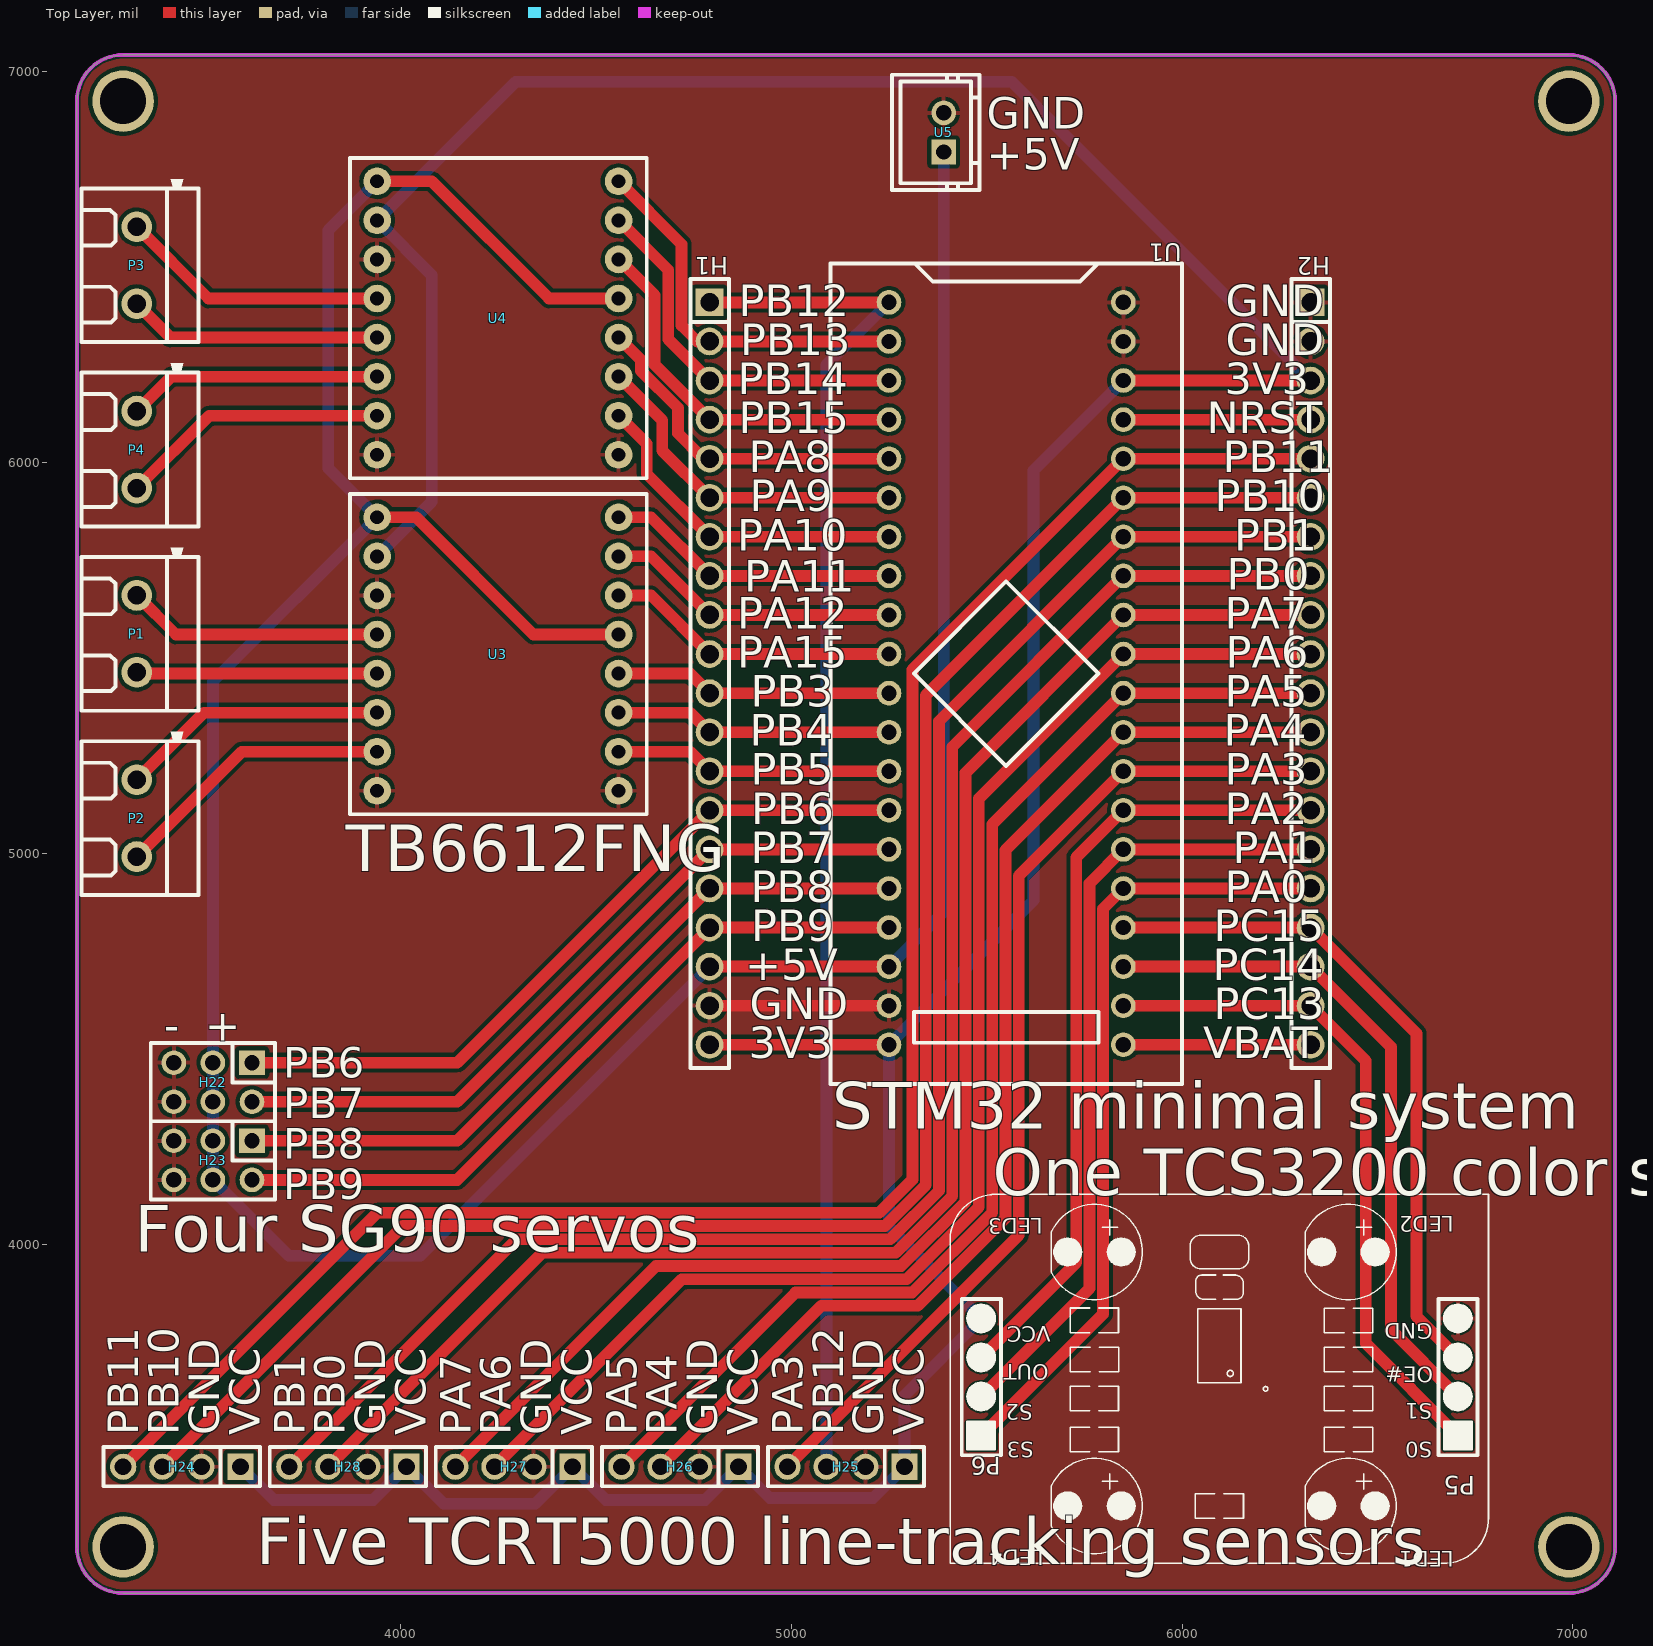
[diagram p0: Top Layer view]
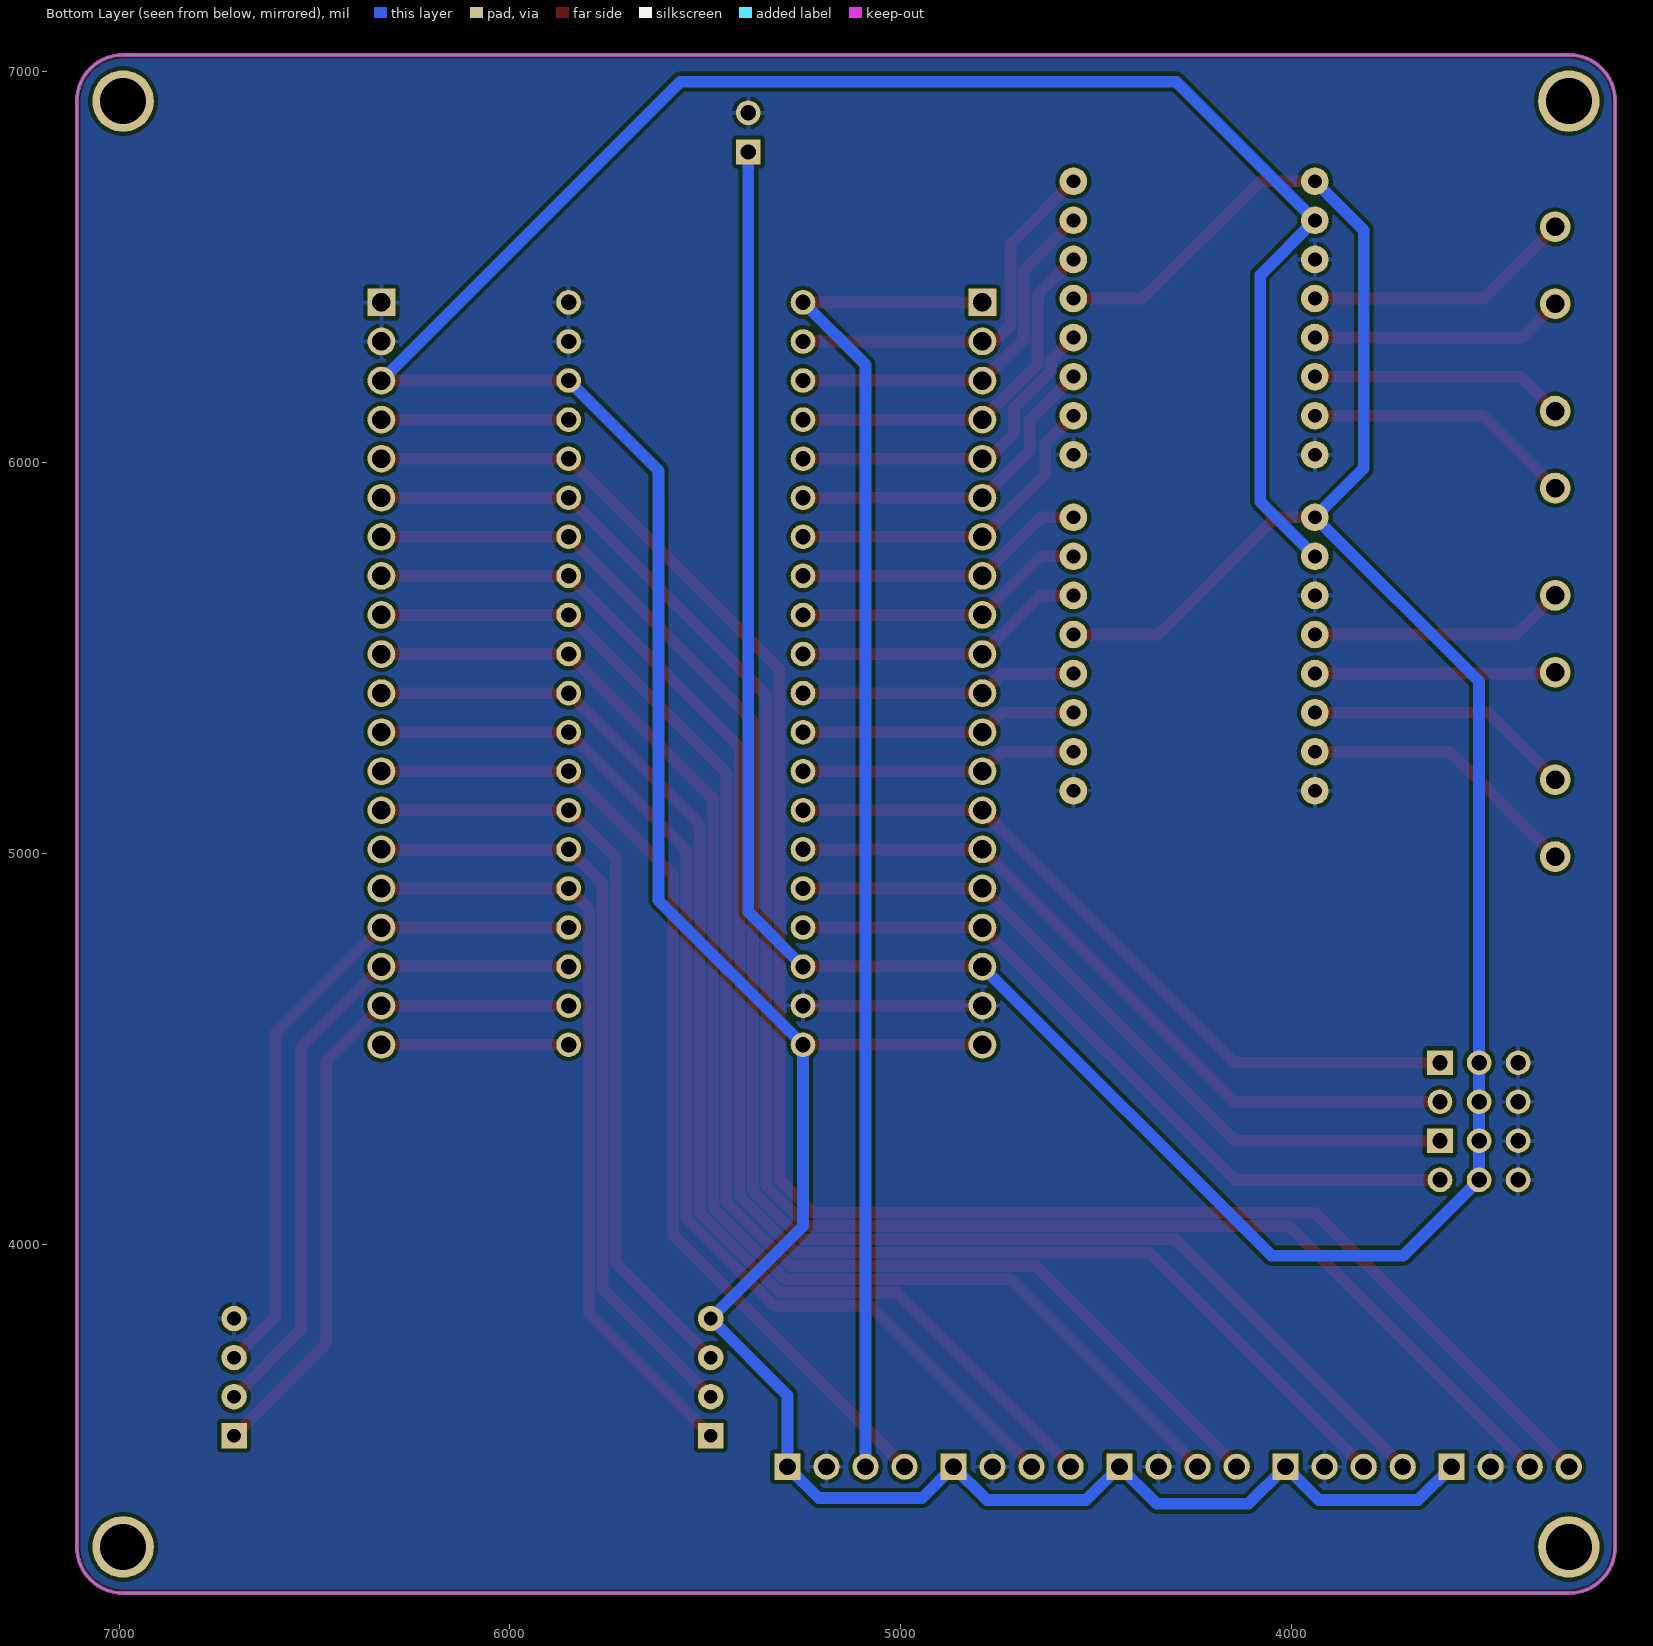
[diagram p1: Bottom Layer view, seen from below]
# Altium PCB MISC88999.pcbdoc
Units mil, origin at the board's own origin, x right, y up, seen from the top; angles counter-clockwise.
Board outline 3937.01 x 3937.01 mil, 2 copper layers (Top Layer, Bottom Layer), stack 62.206 mil thick; 19 components, 45 nets, 166 pads, 0 vias.

## Layer stack, top to bottom
Top Solder Mask Layer: solder mask 0.394, Dk 3.3
Top Layer: signal copper 1.379
Dielectric1: surface 59.449, FR4, Dk 4.5
Bottom Layer: signal copper 1.378
Bottom Solder Mask Layer: solder mask 0.394, Dk 3.3

## Board outline
6990.39,3106.5 ccw(c6990.39,3224.61) 7108.5,3224.61 7108.5,6925.39 ccw(c6990.39,6925.39) 6990.39,7043.5 3289.61,7043.5 ccw(c3289.61,6925.39) 3171.5,6925.39 3171.5,3224.61 ccw(c3289.61,3224.61) 3289.61,3106.5

## Design rules (kind name [scope] priority, off if disabled: settings)
BoardOutlineClearance copperThickness2oz_1 [All] p2 off: genericclearance=7.99 ignorepadtopadclearanceinfootprint=FALSE except(0: Arc-SplitContinuation Track-SplitContinuation SMDPad-SplitContinuation THPad-SplitContinuation Via-SplitContinuation Fill-SplitContinuation Region-SplitContinuation Poly-SplitContinuation Text-SplitContinuation Hole-SplitContinuation; 5.98: Arc-CutoutEdge Track-CutoutEdge SMDPad-CutoutEdge THPad-CutoutEdge Via-CutoutEdge Text-CutoutEdge; 6.9: Hole-OutlineEdge Hole-CutoutEdge; 10: Poly-OutlineEdge Poly-CutoutEdge; 11.81: Arc-OutlineEdge Track-OutlineEdge SMDPad-OutlineEdge THPad-OutlineEdge Via-OutlineEdge Fill-OutlineEdge Region-OutlineEdge Text-OutlineEdge Fill-CutoutEdge Region-CutoutEdge)
BoardOutlineClearance Plane_innerPlane_1 [All] p4 off: genericclearance=4.02 ignorepadtopadclearanceinfootprint=FALSE except(0: Arc-SplitContinuation Track-SplitContinuation SMDPad-SplitContinuation THPad-SplitContinuation Via-SplitContinuation Fill-SplitContinuation Region-SplitContinuation Poly-SplitContinuation Text-SplitContinuation Hole-SplitContinuation; 5.98: Arc-CutoutEdge Track-CutoutEdge SMDPad-CutoutEdge THPad-CutoutEdge Via-CutoutEdge Text-CutoutEdge; 6.9: Hole-OutlineEdge Hole-CutoutEdge; 10: Poly-OutlineEdge Poly-CutoutEdge; 11.81: Arc-OutlineEdge Track-OutlineEdge SMDPad-OutlineEdge THPad-OutlineEdge Via-OutlineEdge Fill-OutlineEdge Region-OutlineEdge Text-OutlineEdge Fill-CutoutEdge Region-CutoutEdge)
BoardOutlineClearance Copper_copperRegion_1 [All] p6 off: genericclearance=4.02 ignorepadtopadclearanceinfootprint=FALSE except(0: Arc-SplitContinuation Track-SplitContinuation SMDPad-SplitContinuation THPad-SplitContinuation Via-SplitContinuation Fill-SplitContinuation Region-SplitContinuation Poly-SplitContinuation Text-SplitContinuation Hole-SplitContinuation; 5.98: Arc-CutoutEdge Track-CutoutEdge SMDPad-CutoutEdge THPad-CutoutEdge Via-CutoutEdge Text-CutoutEdge; 6.9: Hole-OutlineEdge Hole-CutoutEdge; 10: Poly-OutlineEdge Poly-CutoutEdge; 11.81: Arc-OutlineEdge Track-OutlineEdge SMDPad-OutlineEdge THPad-OutlineEdge Via-OutlineEdge Fill-OutlineEdge Region-OutlineEdge Text-OutlineEdge Fill-CutoutEdge Region-CutoutEdge)
BoardOutlineClearance copperThickness1oz_1 [All] p8: genericclearance=4.02 ignorepadtopadclearanceinfootprint=FALSE except(0: Arc-SplitContinuation Track-SplitContinuation SMDPad-SplitContinuation THPad-SplitContinuation Via-SplitContinuation Fill-SplitContinuation Region-SplitContinuation Poly-SplitContinuation Text-SplitContinuation Hole-SplitContinuation; 5.98: Arc-CutoutEdge Track-CutoutEdge SMDPad-CutoutEdge THPad-CutoutEdge Via-CutoutEdge Text-CutoutEdge; 6.9: Hole-OutlineEdge Hole-CutoutEdge; 10: Poly-OutlineEdge Poly-CutoutEdge; 11.81: Arc-OutlineEdge Track-OutlineEdge SMDPad-OutlineEdge THPad-OutlineEdge Via-OutlineEdge Fill-OutlineEdge Region-OutlineEdge Text-OutlineEdge Fill-CutoutEdge Region-CutoutEdge)
Clearance copperThickness2oz [All] p1 off: gap=7.99 ignorepadtopadclearanceinfootprint=FALSE except(5.98: SMDPad-Track SMDPad-SMDPad THPad-Track SMDPad-THPad THPad-THPad Track-Via SMDPad-Via THPad-Via Via-Via Fill-SMDPad Region-SMDPad Fill-THPad Region-THPad Fill-Via Region-Via Fill-Fill Fill-Region Region-Region Arc-Track Arc-SMDPad Arc-THPad Arc-Via Fill-Arc Region-Arc Arc-Arc Text-Track SMDPad-Text Text-THPad Text-Via Fill-Text Region-Text Arc-Text Text-Text; 6.9: Hole-Track Hole-SMDPad Hole-THPad Hole-Via Fill-Hole Region-Hole Hole-Arc Hole-Text; 10: Poly-Track Poly-SMDPad Poly-THPad Poly-Via Poly-Fill Poly-Region Poly-Poly Poly-Arc Poly-Text Poly-Hole; 11.81: Fill-Track Region-Track)
Clearance Plane_innerPlane [All] p3 off: gap=4.02 ignorepadtopadclearanceinfootprint=FALSE except(5.98: SMDPad-Track SMDPad-SMDPad THPad-Track SMDPad-THPad THPad-THPad Track-Via SMDPad-Via THPad-Via Via-Via Fill-SMDPad Region-SMDPad Fill-THPad Region-THPad Fill-Via Region-Via Fill-Fill Fill-Region Region-Region Arc-Track Arc-SMDPad Arc-THPad Arc-Via Fill-Arc Region-Arc Arc-Arc Text-Track SMDPad-Text Text-THPad Text-Via Fill-Text Region-Text Arc-Text Text-Text; 6.9: Hole-Track Hole-SMDPad Hole-THPad Hole-Via Fill-Hole Region-Hole Hole-Arc Hole-Text; 10: Poly-Track Poly-SMDPad Poly-THPad Poly-Via Poly-Fill Poly-Region Poly-Poly Poly-Arc Poly-Text Poly-Hole; 11.81: Fill-Track Region-Track)
Clearance Copper_copperRegion [All] p5 off: gap=4.02 ignorepadtopadclearanceinfootprint=FALSE except(5.98: SMDPad-Track SMDPad-SMDPad THPad-Track SMDPad-THPad THPad-THPad Track-Via SMDPad-Via THPad-Via Via-Via Fill-SMDPad Region-SMDPad Fill-THPad Region-THPad Fill-Via Region-Via Fill-Fill Fill-Region Region-Region Arc-Track Arc-SMDPad Arc-THPad Arc-Via Fill-Arc Region-Arc Arc-Arc Text-Track SMDPad-Text Text-THPad Text-Via Fill-Text Region-Text Arc-Text Text-Text; 6.9: Hole-Track Hole-SMDPad Hole-THPad Hole-Via Fill-Hole Region-Hole Hole-Arc Hole-Text; 10: Poly-Track Poly-SMDPad Poly-THPad Poly-Via Poly-Fill Poly-Region Poly-Poly Poly-Arc Poly-Text Poly-Hole; 11.81: Fill-Track Region-Track)
Clearance copperThickness1oz [All] p7: gap=4.02 ignorepadtopadclearanceinfootprint=FALSE except(5.98: SMDPad-Track SMDPad-SMDPad THPad-Track SMDPad-THPad THPad-THPad Track-Via SMDPad-Via THPad-Via Via-Via Fill-SMDPad Region-SMDPad Fill-THPad Region-THPad Fill-Via Region-Via Fill-Fill Fill-Region Region-Region Arc-Track Arc-SMDPad Arc-THPad Arc-Via Fill-Arc Region-Arc Arc-Arc Text-Track SMDPad-Text Text-THPad Text-Via Fill-Text Region-Text Arc-Text Text-Text; 6.9: Hole-Track Hole-SMDPad Hole-THPad Hole-Via Fill-Hole Region-Hole Hole-Arc Hole-Text; 10: Poly-Track Poly-SMDPad Poly-THPad Poly-Via Poly-Fill Poly-Region Poly-Poly Poly-Arc Poly-Text Poly-Hole; 11.81: Fill-Track Region-Track)
DiffPairsRouting differentialPair [All] p1: maxlimit=6 minlimit=6 mostfreqgap=6 toplayer_minwidth=5 toplayer_prefwidth=10 toplayer_maxwidth=100 toplayer_mingap=6 toplayer_prefgap=6 toplayer_maxgap=6 bottomlayer_minwidth=5 bottomlayer_prefwidth=10 bottomlayer_maxwidth=100 bottomlayer_mingap=6 bottomlayer_prefgap=6 bottomlayer_maxgap=6 maxuncoupledlength=10
HoleToHoleClearance otherClearance [All] p1: gap=11.81 allowstackedmicrovias=TRUE
Length netLength [All] p1: minlimit=0 maxlimit=0
PasteMaskExpansion pasteMaskExpansion [All] p1: expansion=0
PlaneConnect innerPlane [All] p1: planeconnectstyle=Relief reliefexpansion=20 reliefentries=4 reliefconductorwidth=10 reliefairgap=10
PolygonConnect copperRegion [All] p1: connectstyle=Relief reliefconductorwidth=10 reliefentries=4 polygonreliefangle="90 Angle" airgapwidth=10 via.connectstyle=Relief via.reliefconductorwidth=10 via.reliefentries=4 via.polygonreliefangle="90 Angle" via.airgapwidth=10
RoutingVias viaSize [All] p1: holewidth=12.01 width=24.02 viastyle="Through Hole" minholewidth=11.81 minwidth=19.68 maxholewidth=248.03 maxwidth=393.7
SolderMaskExpansion solderMaskExpansion [IsVia] p1: expansion=-1000 istentingtop=TRUE
SolderMaskExpansion solderMaskExpansion [All] p2: expansion=2 istentingtop=FALSE
Width copperThickness2oz_2 [All] p1 off: maxlimit=100 minlimit=8 preferedwidth=10
Width copperThickness1oz_2 [All] p2: maxlimit=100 minlimit=5 preferedwidth=10

## Components (designator, comment, footprint, x,y, rotation, side; value= is the part's Value field where it differs from the comment)
H1 "" HDR-TH_20P-P2.54-V-F 4790.84,5460 r270 top
H2 "" HDR-TH_20P-P2.54-V-F 6329.05,5460 r270 top
H22 "" HDR-TH_6P-P2.54-V-F-R2-C3-S2.54 3519.7,4414.1 r180 top
H23 "" HDR-TH_6P-P2.54-V-F-R2-C3-S2.54 3519.7,4214.1 r180 top
H24 "" HDR-TH_4P-P2.54-V-M 3440,3430 r180 top
H25 "" HDR-TH_4P-P2.54-V-M 5140,3430 r180 top
H26 "" HDR-TH_4P-P2.54-V-M 4715,3430 r180 top
H27 "" HDR-TH_4P-P2.54-V-M 4290,3430 r180 top
H28 "" HDR-TH_4P-P2.54-V-M 3865,3430 r180 top
P1 "KF301-2P terminal block" CONN-TH_XY301V-A-5.0-2P 3325,5561.67 r90 top
P2 "KF301-2P terminal block" CONN-TH_XY301V-A-5.0-2P 3325,5090 r90 top
P3 "KF301-2P terminal block" CONN-TH_XY301V-A-5.0-2P 3325,6505 r90 top
P4 "KF301-2P terminal block" CONN-TH_XY301V-A-5.0-2P 3325,6033.33 r90 top
P5 "2.54-1*4P_JX" 2.54-1*4P_JX 6706.22,3659.3 r90 top
P6 "2.54-1*4P_JX" 2.54-1*4P_JX 5486.22,3659.3 r90 top
U1 "STM32F103C8T6-Card" CONN-TH_L53.3-W22.9_STM32F103C8T6-CARD 5550,5460 r270 top
U3 "" tb6612 3940,5860 r0 top
U4 "" tb6612 3940,6720 r0 top
U5 "_x001F_XH2.54-2P" CONN-TH_2P-P2.54-V 5390,6845 r90 top

## Footprints (in the part's own frame and the unit in brackets; to place one, negate y for a bottom-side part, rotate by r counter-clockwise, add the part's x,y. Pads: shape width x height; smd on the part's side, far side on the other; paste and mask are expansions set on the pad)
2.54-1*4P_JX [mil]
  rect 65x65 hole 35 paste+0 mask+4: 1(-150,0)
  round 65 hole 35 paste+0 mask+4: 2(-50,0) 3(50,0) 4(150,0)
  silkscreen extent -200,-50 200,50
CONN-TH_2P-P2.54-V [mm]
  rect 1.6x1.6 hole 1: 1(-1.27,0)
  round 1.6 hole 1: 2(1.27,0)
  silkscreen extent -3.75,-2.34 3.75,3.36
CONN-TH_L53.3-W22.9_STM32F103C8T6-CARD [mm]
  round 1.6 hole 1: 1(-24.13,-7.62) 2(-21.59,-7.62) 3(-19.05,-7.62) 4(-16.51,-7.62) 5(-13.97,-7.62) 6(-11.43,-7.62) 7(-8.89,-7.62) 8(-6.35,-7.62) 9(-3.81,-7.62) 10(-1.27,-7.62) 11(1.27,-7.62) 12(3.81,-7.62) 13(6.35,-7.62) 14(8.89,-7.62) 15(11.43,-7.62) 16(13.97,-7.62) 17(16.51,-7.62) 18(19.05,-7.62) 19(21.59,-7.62) 20(24.13,-7.62) 21(24.13,7.62) 22(21.59,7.62) 23(19.05,7.62) 24(16.51,7.62) 25(13.97,7.62) 26(11.43,7.62) 27(8.89,7.62) 28(6.35,7.62) 29(3.81,7.62) 30(1.27,7.62) 31(-1.27,7.62) 32(-3.81,7.62) 33(-6.35,7.62) 34(-8.89,7.62) 35(-11.43,7.62) 36(-13.97,7.62) 37(-16.51,7.62) 38(-19.05,7.62) 39(-21.59,7.62) 40(-24.13,7.62)
  silkscreen extent -26.67,-11.43 26.67,11.43
CONN-TH_XY301V-A-5.0-2P [mm]
  round 2 hole 1.2: 1(-2.5,0) 2(2.5,0)
  silkscreen extent -5,-4 5.6,3.6
HDR-TH_4P-P2.54-V-M [mm]
  rect 1.7x1.7 hole 1.1: 1(-3.81,0)
  round 1.7 hole 1.1: 2(-1.27,0) 3(1.27,0) 4(3.81,0)
  silkscreen extent -5.08,-1.27 5.08,1.27
HDR-TH_6P-P2.54-V-F-R2-C3-S2.54 [mm]
  rect 1.7x1.6 hole 1: 1(-2.54,-1.27)
  round 1.6 hole 1: 2(-2.54,1.27) 3(0,-1.27) 4(0,1.27) 5(2.54,-1.27) 6(2.54,1.27)
  silkscreen extent -4.04,-2.54 4.04,2.54
HDR-TH_20P-P2.54-V-F [mm]
  rect 1.8x1.8 hole 1.2: 1(-24.13,0)
  round 1.8 hole 1.2: 2(-21.59,0) 3(-19.05,0) 4(-16.51,0) 5(-13.97,0) 6(-11.43,0) 7(-8.89,0) 8(-6.35,0) 9(-3.81,0) 10(-1.27,0) 11(1.27,0) 12(3.81,0) 13(6.35,0) 14(8.89,0) 15(11.43,0) 16(13.97,0) 17(16.51,0) 18(19.05,0) 19(21.59,0) 20(24.13,0)
  silkscreen extent -25.65,-1.25 25.65,1.25
tb6612 [mm]
  round 1.8 hole 0.9: 1(0,0) 2(0,-2.54) 3(0,-5.08) 4(0,-7.62) 5(0,-10.16) 6(0,-12.7) 7(0,-15.24) 8(0,-17.78) 9(15.697,-17.78) 10(15.697,-15.24) 11(15.697,-12.7) 12(15.697,-10.16) 13(15.697,-7.62) 14(15.697,-5.08) 15(15.697,-2.54) 16(15.697,0)
  silkscreen extent -1.78,-19.3 17.53,1.52

## Free pads (board coordinates)
  round 157.48 hole 118.11: 1(3289.61,6925.39) 1(3289.61,3224.61) 1(6990.39,6925.39) 1(6990.39,3224.61)

## Nets (pads, with @x,y where several pads share a name; then routed paths per layer and width w, separated by ;. In a path a pad name is that pad's centre, name@x,y a point inside that pad or via, vN(x,y) a via of type N, cw(c..) or ccw(c..) an arc to the next point about the centre after c; other vN are vias at no path point)
$1N16642: P2.1 U3.7 | length 726.2
  Top Layer w30: P2.1 3593.43,5260 U3.7
$1N16644: P2.2 U3.6 | length 686.1
  Top Layer w30: P2.2 3496.57,5360 U3.6
$1N16646: P1.1 U3.5 | length 616.3
  Top Layer w30: P1.1 3328.24,5460 U3.5
$1N16648: P1.2 U3.4 | length 656.5
  Top Layer w30: P1.2 3425.09,5560 U3.4
$1N17933: P4.1 U4.7 | length 691.7
  Top Layer w30: P4.1 3510.09,6120 U4.7
$1N17941: P4.2 U4.6 | length 651.6
  Top Layer w30: P4.2 3413.24,6220 U4.6
$1N17944: P3.1 U4.5 | length 650.9
  Top Layer w30: P3.1 3411.57,6320 U4.5
$1N17948: P3.2 U4.4 | length 691
  Top Layer w30: P3.2 3508.43,6420 U4.4
+5V: H1.18 H22.3 H22.4 H23.3 H23.4 U1.18 U3.1 U3.13 U4.1 U4.13 U5.1 | length 8578.3
  Top Layer w30: U3.1 4040,5860 4340,5560 U3.13 ; U4.1 4080,6720 4380,6420 U4.13 ; H1.18 U1.18
  Bottom Layer w30: U4.1 3815,6595 3815,5985 U3.1 3519.7,5439.7 H22.3 H22.4 H23.3 H23.4 3713.8,3970 4050.84,3970 H1.18 ; U1.18 5390,4850 U5.1
GND: H1.19 H2.1 H2.2 H22.5 H22.6 H23.5 H23.6 H24.2 H25.2 H26.2 H27.2 H28.2 P5.4 U1.19 U1.39 U1.40 U3.3 U3.8 U3.9 U4.3 U4.8 U4.9 U5.2 | length 459.2
  Top Layer w30: H1.19 U1.19
NRST: H2.4 U1.37 | length 479
  Top Layer w30: U1.37 H2.4
PA0: H2.16 P6.1 U1.25 | length 2030.4
  Top Layer w30: P6.1 5797.52,3820.6 5797.52,4857.52 U1.25 H2.16
PA1: H2.15 P6.2 U1.26 | length 2030.4
  Top Layer w30: P6.2 5763.51,3886.58 5763.51,4923.5 U1.26 H2.15
PA2: H2.14 P6.3 U1.27 | length 2030.4
  Top Layer w30: P6.3 5729.49,3952.57 5729.49,4989.49 U1.27 H2.14
PA3: H2.13 H25.4 U1.28 | length 2615.3
  Top Layer w30: H25.4 5582.13,4022.13 5582.13,4942.12 U1.28 H2.13
PA4: H2.12 H26.3 U1.29 | length 2994.4
  Top Layer w30: H26.3 5076.89,3841.89 5323.63,3841.89 5548.11,4066.37 5548.11,5008.11 U1.29 H2.12
PA5: H2.11 H26.4 U1.30 | length 3166.2
  Top Layer w30: H26.4 5010.91,3875.91 5309.54,3875.91 5514.09,4080.46 5514.09,5074.09 U1.30 H2.11
PA6: H2.10 H27.3 U1.31 | length 3563.1
  Top Layer w30: H27.3 4719.92,3909.92 5295.45,3909.92 5480.08,4094.55 5480.08,5140.08 U1.31 H2.10
PA7: H2.9 H27.4 U1.32 | length 3734.9
  Top Layer w30: H27.4 4653.94,3943.94 5281.36,3943.94 5446.06,4108.64 5446.06,5206.06 U1.32 H2.9
PA8: H1.5 U1.5 U4.12 | length 874.9
  Top Layer w30: U4.12 4615,6263 4615,6235 4710,6140 4710,6075 4775,6010 H1.5 U1.5
PA9: H1.6 U1.6 U4.11 | length 865.6
  Top Layer w30: U4.11 4670,6108 4670,6030.84 H1.6 U1.6
PA10: H1.7 U1.7 U4.10 | length 865.6
  Top Layer w30: U4.10 4630,6048 4630,5970.84 H1.7 U1.7
PA11: H1.8 U1.8 U3.16 | length 754.1
  Top Layer w30: U3.16 4640.84,5860 H1.8 U1.8
PA12: H1.9 U1.9 U3.15 | length 754.1
  Top Layer w30: U3.15 4640.84,5760 H1.9 U1.9
PA15: H1.10 U1.10 U3.14 | length 754.1
  Top Layer w30: U3.14 4640.84,5660 H1.10 U1.10
PB0: H2.8 H28.3 U1.33 | length 4131.7
  Top Layer w30: H28.3 4362.95,3977.95 5267.27,3977.95 5412.05,4122.73 5412.05,5272.04 U1.33 H2.8
PB1: H2.7 H28.4 U1.34 | length 4303.5
  Top Layer w30: H28.4 4296.97,4011.97 5253.18,4011.97 5378.03,4136.82 5378.03,5338.03 U1.34 H2.7
PB3: H1.11 U1.11 U3.12 | length 712.7
  Top Layer w30: U3.12 4740.84,5460 H1.11 U1.11
PB4: H1.12 U1.12 U3.11 | length 712.7
  Top Layer w30: U3.11 4740.84,5360 H1.12 U1.12
PB5: H1.13 U1.13 U3.10 | length 712.7
  Top Layer w30: U3.10 4740.84,5260 H1.13 U1.13
PB6: H1.14 H22.1 U1.14 | length 1897.8
  Top Layer w30: H22.1 4144.94,4464.1 H1.14 U1.14
PB7: H1.15 H22.2 U1.15 | length 1897.8
  Top Layer w30: H22.2 4144.94,4364.1 H1.15 U1.15
PB8: H1.16 H23.1 U1.16 | length 1897.8
  Top Layer w30: H23.1 4144.94,4264.1 H1.16 U1.16
PB9: H1.17 H23.2 U1.17 | length 1897.8
  Top Layer w30: H23.2 4144.94,4164.1 H1.17 U1.17
PB10: H2.6 H24.3 U1.35 | length 4700.3
  Top Layer w30: H24.3 4005.98,4045.98 5239.09,4045.98 5344.02,4150.91 5344.02,5404.01 U1.35 H2.6
PB11: H2.5 H24.4 U1.36 | length 4872.2
  Top Layer w30: H24.4 3940,4080 5225,4080 5310,4165 5310,5470 U1.36 H2.5
PB12: H1.1 H25.3 U1.1 | length 3505.4
  Top Layer w30: H1.1 U1.1
  Bottom Layer w30: H25.3 5090,6250 U1.1
PB13: H1.2 U1.2 U4.16 | length 983.7
  Top Layer w30: U4.16 4719.02,6558.98 4719.02,6350.98 4760,6310 H1.2 U1.2
PB14: H1.3 U1.3 U4.15 | length 965.6
  Top Layer w30: U4.15 4685,6493 4685,6315.84 H1.3 U1.3
PB15: H1.4 U1.4 U4.14 | length 965.6
  Top Layer w30: U4.14 4650,6428 4650,6250.84 H1.4 U1.4
PC13: H2.19 P5.1 U1.22 | length 1736
  Top Layer w30: U1.22 H2.19 6470,4469.05 6470,3745.51 P5.1
PC14: H2.18 P5.2 U1.23 | length 1736
  Top Layer w30: U1.23 H2.18 6535,4504.05 6535,3780.51 P5.2
PC15: H2.17 P5.3 U1.24 | length 1736
  Top Layer w30: U1.24 H2.17 6600,4539.05 6600,3815.51 P5.3
VBAT: H2.20 U1.21 | length 479
  Top Layer w30: U1.21 H2.20
VCC: H1.20 H2.3 H24.1 H25.1 H26.1 H27.1 H28.1 P6.4 U1.20 U1.38 U3.2 U4.2 | length 9960.6
  Top Layer w30: H1.20 U1.20 ; U1.38 H2.3
  Bottom Layer w30: H24.1 3675,3345 3930,3345 H28.1 4110,3335 4345,3335 H27.1 4525,3345 4780,3345 H26.1 4945,3350 5210,3350 H25.1 5290,3613.08 P6.4 5250,4045.51 U1.20 5620,4880 5620,5980 U1.38 ; U3.2 4080,5900 4080,6480 U4.2 4295,6975 5564.05,6975 H2.3

## Polygon pours and split planes (outlines as drawn)
GND on Bottom Layer (solid, remove dead copper, pour order 2): 3100,7165 3100,3000 7275,3000 7275,7165
GND on Top Layer (solid, remove dead copper, pour order 0): 3000,7145 3000,3075 7385,3075 7385,7145

## Keep-outs
Board Outline Layer:
  the board outline again, w10

## Silkscreen, mask and mechanical layers (free items; w line width, h text height)
Top Silkscreen Layer:
  drawing of 188 lines, arcs and shapes, not listed
  text "GND" at 5500,6855 h80
  text "+5V" at 5500,6750 h80
  text "PB12" at 4865.64,6375 h80
  text "GND" at 6111.65,6375 h80
  text "PB13" at 4868.85,6275 h80
  text "GND" at 6111.65,6275 h80
  text "PB14" at 4863.34,6175 h80
  text "3V3" at 6109.45,6175 h80
  text "PB15" at 4865.64,6075 h80
  text "NRST" at 6063.65,6075 h80
  text "PA8" at 4891.24,5975 h80
  text "PB11" at 6104.05,5975 h80
  text "PA9" at 4893.44,5875 h80
  text "PB10" at 6083.85,5875 h80
  text "PA10" at 4861.14,5775 h80
  text "PB1" at 6134.15,5775 h80
  text "PB0" at 6113.95,5675 h80
  text "PA11" at 4879.55,5670 h80
  text "PA12" at 4861.14,5575 h80
  text "PA7" at 6109.45,5575 h80
  text "PA15" at 4861.14,5475 h80
  text "PA6" at 6111.65,5475 h80
  text "PB3" at 4895.74,5375 h80
  text "PA5" at 6109.45,5375 h80
  text "PB4" at 4893.44,5275 h80
  text "PA4" at 6107.15,5275 h80
  text "PB5" at 4895.74,5175 h80
  text "PA3" at 6109.45,5175 h80
  text "PB6" at 4897.94,5075 h80
  text "PA2" at 6109.45,5075 h80
  text "PB7" at 4895.74,4975 h80
  text "PA1" at 6129.65,4975 h80
  text "TB6612FNG" at 3860,4953.99 h120
  text "PB8" at 4895.74,4875 h80
  text "PA0" at 6109.45,4875 h80
  text "PB9" at 4897.94,4775 h80
  text "PC15" at 6081.55,4775 h80
  text "+5V" at 4882.24,4675 h80
  text "PC14" at 6079.25,4675 h80
  text "GND" at 4893.44,4575 h80
  text "PC13" at 6081.55,4575 h80
  text "-" at 3395,4519.9 h78.74
  text "+" at 3500,4520 h78.74
  text "3V3" at 4891.24,4475 h80
  text "VBAT" at 6054.65,4475 h80
  text "PB6" at 3700,4425 h78.74
  text "PB7" at 3700,4321.67 h78.74
  text "STM32 minimal system" at 5105,4295 h120
  text "PB8" at 3700,4218.33 h78.74
  text "One TCS3200 color sensor" at 5515,4125 h120
  text "PB9" at 3700,4115 h78.74
  text "LED2" at 6695.5,4070.77 h39.37 r180
  text "LED3" at 5643.8,4065.77 h39.37 r180
  text "Four SG90 servos" at 3320,3980 h120
  text "GND" at 6642.2,3797.76 h39.37 r180
  text "VCC" at 5663.9,3789.36 h39.37 r180
  text "OUT" at 5658.7,3691.66 h39.37 r180
  text "OE#" at 6642.9,3685.96 h39.37 r180
  text "S1" at 6640.9,3591.96 h39.37 r180
  text "S2" at 5617.6,3589.36 h39.37 r180
  text "PB11" at 3329.1,3510.3 h78.74 r90
  text "PB10" at 3432.43,3510.3 h78.74 r90
  text "GND" at 3535.76,3510.3 h78.74 r90
  text "VCC" at 3639.1,3510.3 h78.74 r90
  text "PB1" at 3754.1,3510.3 h78.74 r90
  text "PB0" at 3857.43,3510.3 h78.74 r90
  text "GND" at 3960.76,3510.3 h78.74 r90
  text "VCC" at 4064.1,3510.3 h78.74 r90
  text "PA7" at 4179.1,3510.3 h78.74 r90
  text "PA6" at 4282.43,3510.3 h78.74 r90
  text "GND" at 4385.76,3510.3 h78.74 r90
  text "VCC" at 4489.1,3510.3 h78.74 r90
  text "PA5" at 4604.1,3510.3 h78.74 r90
  text "PA4" at 4707.43,3510.3 h78.74 r90
  text "GND" at 4810.76,3510.3 h78.74 r90
  text "VCC" at 4914.1,3510.3 h78.74 r90
  text "PA3" at 5029.1,3510.3 h78.74 r90
  text "PB12" at 5132.43,3510.3 h78.74 r90
  text "GND" at 5235.76,3510.3 h78.74 r90
  text "VCC" at 5339.1,3510.3 h78.74 r90
  text "S3" at 5620.2,3493.76 h39.37 r180
  text "S0" at 6640.9,3493.96 h39.37 r180
  text "LED4" at 5645.9,3216.86 h39.37 r180
  text "LED1" at 6695.8,3213.56 h39.37 r180
  text "Five TCRT5000 line-tracking sensors" at 3630,3180 h120